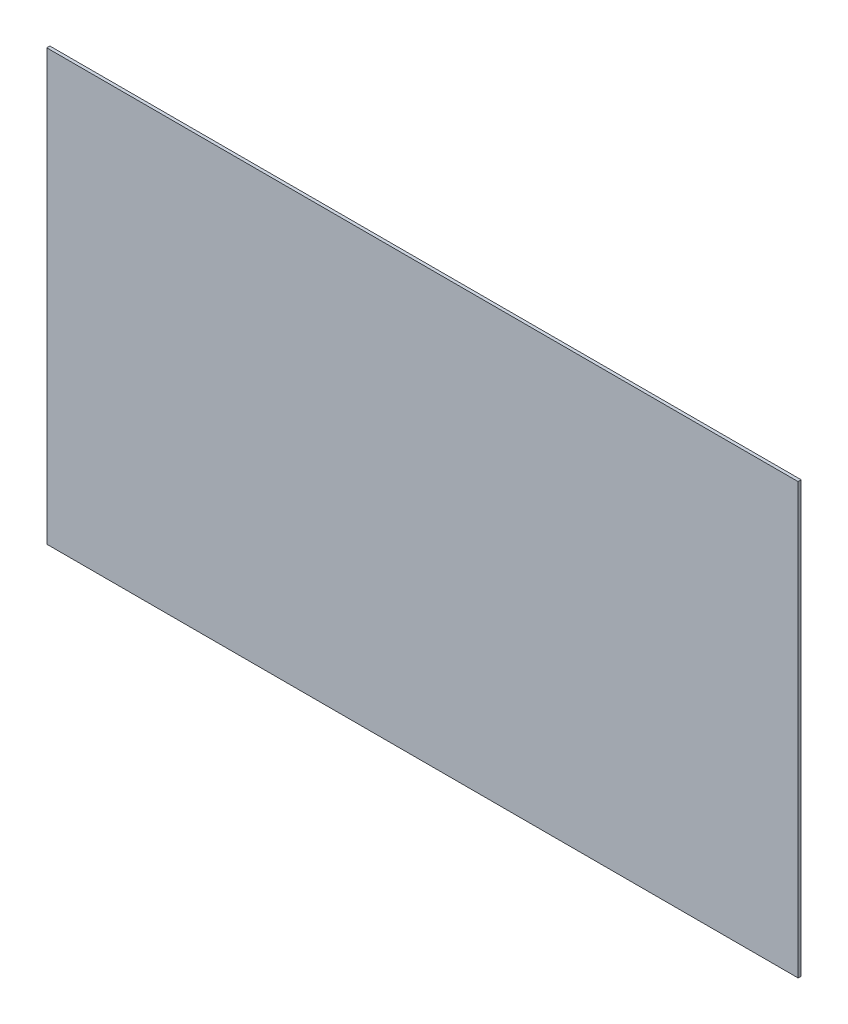
SolidWorks part; units mm, degrees
material "PMMA(有机玻璃)"
ref_plane "前视" through (0, 0, 0) normal (0, 0, 1) x (1, 0, 0)
ref_plane "上视" through (0, 0, 0) normal (0, 1, 0) x (1, 0, 0)
ref_plane "右视" through (0, 0, 0) normal (1, 0, 0) x (0, 0, -1)
sketch "草图1" plane through (0, 0, 0) normal (0, 0, 1) x (1, 0, 0)
  line L1 (-603, 345) -> (603, 345)
  line L2 (-603, 345) -> (-603, -345)
  line L3 (-603, -345) -> (603, -345)
  line L4 (603, 345) -> (603, -345)
  line L5 (-603, 345) -> (603, -345) construction
  line L6 (-603, -345) -> (603, 345) construction
  point P0 (0, 0)
  dimension "D1" = 690
  dimension "D2" = 1206
extrude "凸台-拉伸1" add sketch "草图1" along normal blind 5
hole_wizard "M5 间隙孔1" positions "草图3" profile "草图2" hole size "M5" standard "GB"
sketch "草图3" plane through (0, 0, 5) normal (0, 0, 1) x (1, 0, 0)
  line L0 (-427.5, 273) -> (-427.5, -273) construction
  line L1 (-427.5, -273) -> (427.5, -273) construction
  line L2 (0, 273) -> (0, -273) construction
  line L3 (427.5, 273) -> (-427.5, 273) construction
  line L5 (-427.5, 0) -> (427.5, 0) construction
  line L6 (427.5, -273) -> (427.5, 273) construction
  point P0 (-375, -261)
  point P46 (415.5, 250)
  point P48 (-415.5, 250)
  point P58 (-125, -261)
  point P59 (125, -261)
  point P61 (-125, 261)
  point P62 (125, 261)
  point P64 (-375, 261)
  point P88 (375, -261)
  point P89 (375, 261)
  point P108 (415.5, 0)
  point P109 (-415.5, 0)
  point P110 (415.5, -250)
  point P111 (-415.5, -250)
  dimension "D1" = 12
  dimension "D2" = 12
  dimension "D5" = 3
  dimension "D3" = 12
  dimension "D6" = 4
  dimension "D4" = 2
sketch "草图2" plane through (-375, -261, 5) normal (1, 0, 0) x (0, -1, 0)
  line L0 (0, 0) -> (0, 5)
  line L1 (0, 5) -> (2.75, 5)
  line L2 (2.75, 5) -> (2.75, 0)
  line L5 (2.75, 0) -> (0, 0)
  line L11 (0, -6.35) -> (0, 107.95) construction
  dimension "通孔孔直径" = 5.5
  dimension "通孔孔深度" = 5
